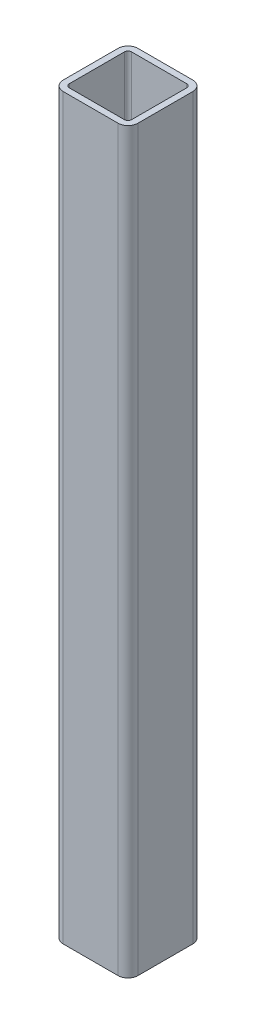
from build123d import *

# Parameters (mm, degrees)
GB_T6728_2002_120_120_10_1_DEPTH = 1185


with BuildPart() as part:
    # Sketch12 → 结构用冷弯空心方钢(gb t6728-2002) 120×120×10(1) (new body)
    with BuildSketch(Plane(origin=(0, 0, 0), x_dir=(-1, 0, 0), z_dir=(0, 1, 0))):
        with BuildLine():
            Line((-44, -60), (44, -60))
            ThreePointArc((44, -60), (55.313708499, -55.313708499), (60, -44))
            Line((60, -44), (60, 44))
            ThreePointArc((60, 44), (55.313708499, 55.313708499), (44, 60))
            Line((44, 60), (-44, 60))
            ThreePointArc((-44, 60), (-55.313708499, 55.313708499), (-60, 44))
            Line((-60, 44), (-60, -44))
            ThreePointArc((-60, -44), (-55.313708499, -55.313708499), (-44, -60))
        make_face()
        with BuildLine():
            Line((-44, -50), (44, -50))
            ThreePointArc((44, -50), (48.242640687, -48.242640687), (50, -44))
            Line((50, -44), (50, 44))
            ThreePointArc((50, 44), (48.242640687, 48.242640687), (44, 50))
            Line((44, 50), (-44, 50))
            ThreePointArc((-44, 50), (-48.242640687, 48.242640687), (-50, 44))
            Line((-50, 44), (-50, -44))
            ThreePointArc((-50, -44), (-48.242640687, -48.242640687), (-44, -50))
        make_face(mode=Mode.SUBTRACT)
    extrude(amount=GB_T6728_2002_120_120_10_1_DEPTH)


solid = part.part
